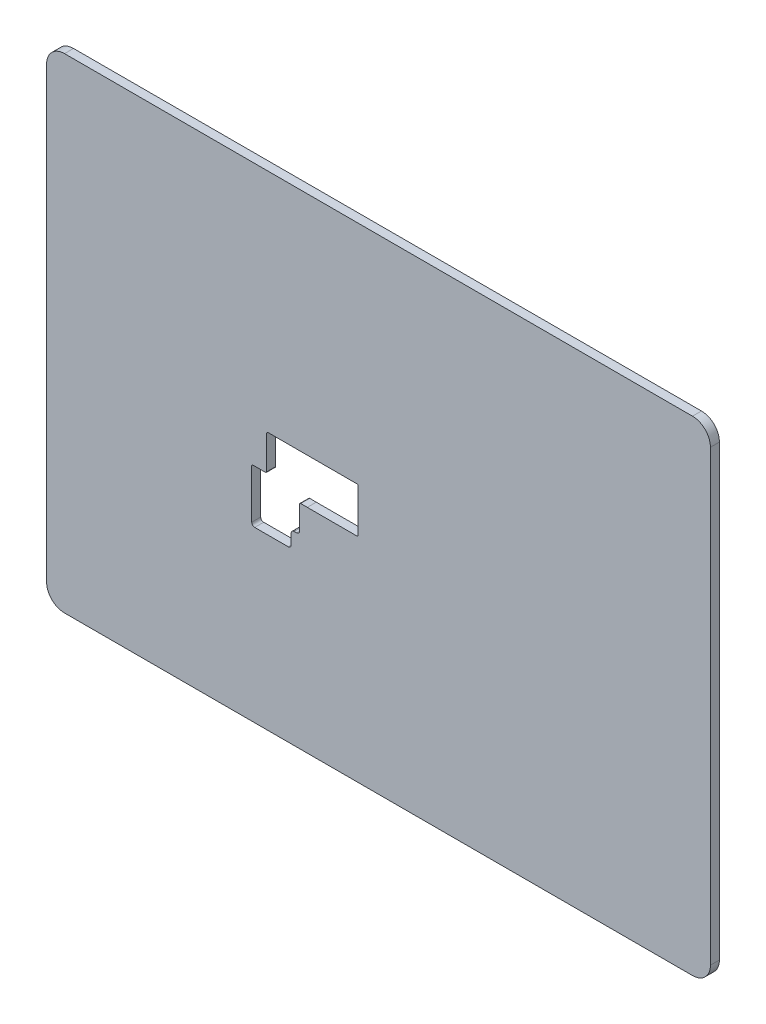
from build123d import *

# Parameters (mm, degrees)
EXTRUDE_1_DEPTH     = 15
CUT_EXTRUDE_1_DEPTH = 829.113419972


with BuildPart() as part:
    # 草图1 → 凸台-拉伸1 (new body)
    with BuildSketch(Plane.XY):
        with BuildLine():
            Line((-456.754393923, 478.74061611), (-456.754393923, -271.25938389))
            ThreePointArc((-456.754393923, -271.25938389), (-447.967597359, -292.472587326), (-426.754393923, -301.25938389))
            Line((-426.754393923, -301.25938389), (623.245606077, -301.25938389))
            ThreePointArc((623.245606077, -301.25938389), (644.458809512, -292.472587326), (653.245606077, -271.25938389))
            Line((653.245606077, -271.25938389), (653.245606077, 478.74061611))
            ThreePointArc((653.245606077, 478.74061611), (644.458809512, 499.953819545), (623.245606077, 508.74061611))
            Line((623.245606077, 508.74061611), (-426.754393923, 508.74061611))
            ThreePointArc((-426.754393923, 508.74061611), (-447.967597359, 499.953819545), (-456.754393923, 478.74061611))
        make_face()
    extrude(amount=EXTRUDE_1_DEPTH)

    # 草图2 → 切除-拉伸1 (cut, through all)
    with BuildSketch(Plane.XY.offset(15)):
        with BuildLine():
            Line((-113.754393923, 51.678144789), (-113.754393923, -13.321855211))
            ThreePointArc((-113.754393923, -13.321855211), (-112.289927829, -16.857389117), (-108.754393923, -18.321855211))
            Line((-108.754393923, -18.321855211), (-52.754393923, -18.321855211))
            ThreePointArc((-52.754393923, -18.321855211), (-49.218860017, -16.857389117), (-47.754393923, -13.321855211))
            Line((-47.754393923, -13.321855211), (-47.754393923, 3.746846437))
            ThreePointArc((-47.754393923, 3.746846437), (-46.31430038, 7.257838606), (-42.823567517, 8.746367915))
            Line((-42.823567517, 8.746367915), (-38.68522033, 8.803626264))
            ThreePointArc((-38.68522033, 8.803626264), (-35.194487466, 10.292155573), (-33.754393923, 13.803147743))
            Line((-33.754393923, 13.803147743), (-33.754393923, 51.678144789))
            Line((-33.754393923, 51.678144789), (-33.754393923, 53.24152579))
            ThreePointArc((-33.754393923, 53.24152579), (-33.016130918, 54.337823849), (-31.755279488, 54.734252116))
            Line((-31.755279488, 54.734252116), (-20.864600558, 54.67610792))
            Line((-20.864600558, 54.67610792), (62.197064842, 54.67610792))
            ThreePointArc((62.197064842, 54.67610792), (63.611278404, 55.261894358), (64.197064842, 56.67610792))
            Line((64.197064842, 56.67610792), (64.197064842, 89.975586232))
            Line((64.197064842, 89.975586232), (64.197064842, 128.216032673))
            ThreePointArc((64.197064842, 128.216032673), (63.611278404, 129.630246236), (62.197064842, 130.216032673))
            Line((62.197064842, 130.216032673), (-86.692151935, 130.216032673))
            ThreePointArc((-86.692151935, 130.216032673), (-88.106365497, 129.630246236), (-88.692151935, 128.216032673))
            Line((-88.692151935, 128.216032673), (-88.692151935, 100.216032673))
            Line((-88.692151935, 100.216032673), (-88.692151935, 72.429613021))
            ThreePointArc((-88.692151935, 72.429613021), (-89.277938372, 71.015399459), (-90.692151935, 70.429613021))
            Line((-90.692151935, 70.429613021), (-111.754393923, 70.429613021))
            ThreePointArc((-111.754393923, 70.429613021), (-113.168607486, 69.843826583), (-113.754393923, 68.429613021))
            Line((-113.754393923, 68.429613021), (-113.754393923, 51.678144789))
        make_face()
    extrude(amount=-CUT_EXTRUDE_1_DEPTH, mode=Mode.SUBTRACT)


solid = part.part
